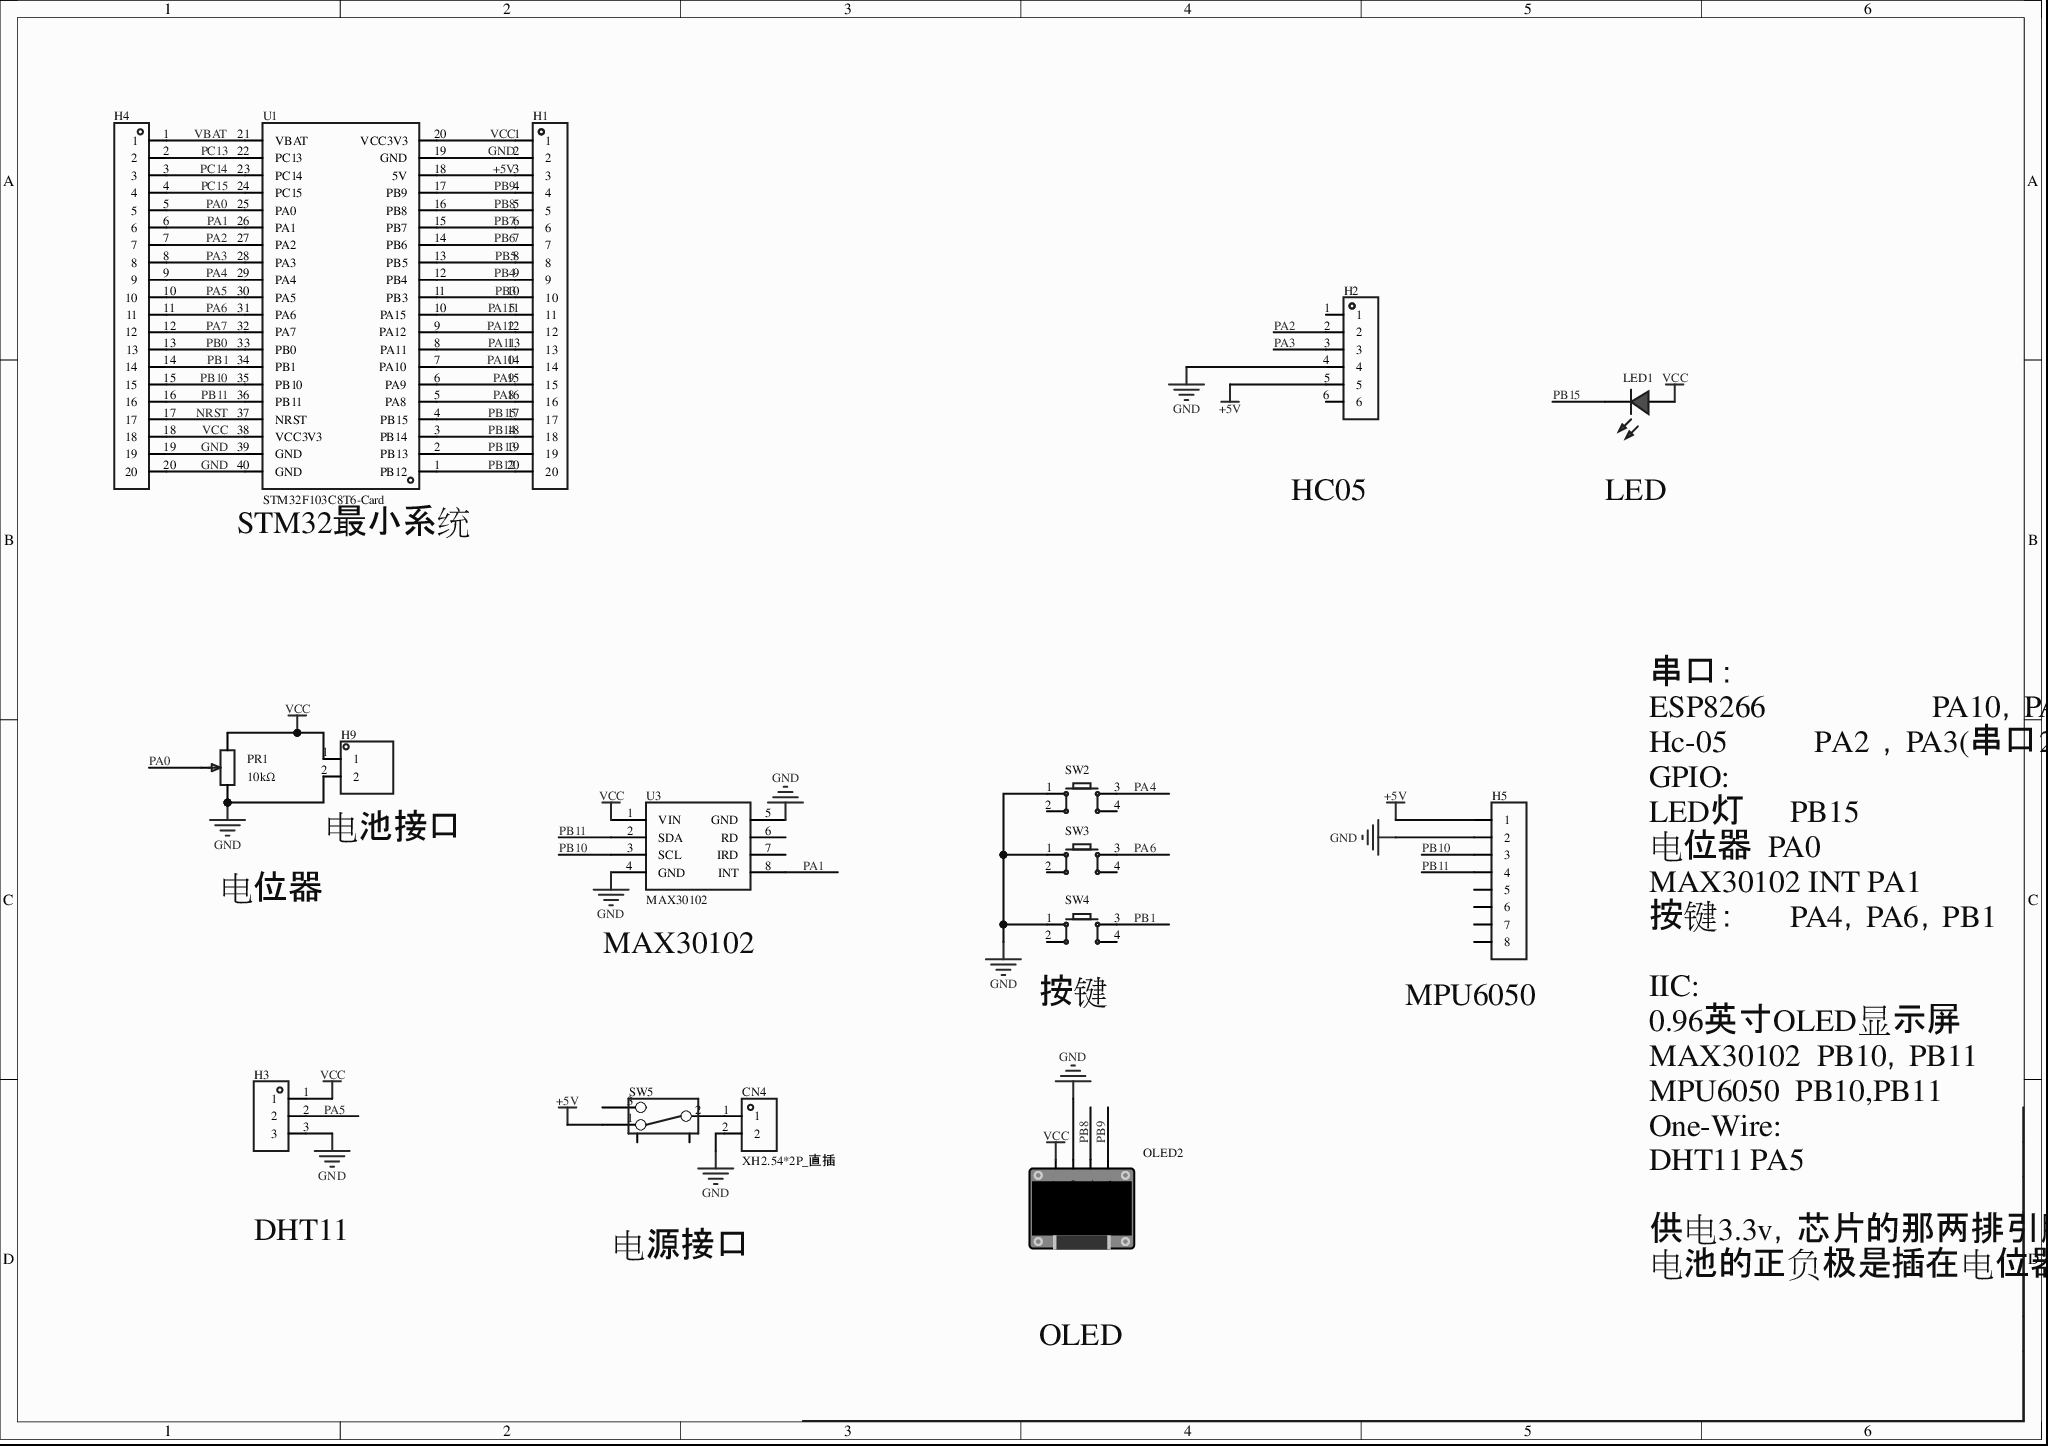
[diagram p0: MISC51261-3.schdoc]
# Altium project MISC51261-2.PrjPcb
1 sheet, 16 parts. Net scope: global (net labels, ports and power ports of the same name join across sheets).
Board file: MISC51261.pcbdoc

## Sheet MISC51261-3.schdoc
size 297 x 209 mm; Version: V1.0; @Project Name: MISC51261; @Page Count: 1; @Update Date: 2026-05-06; @Create Date: 2026-05-06; @Schematic Name: MISC51261; @Page No: 1; @Create Time: 23:22:16; @Update Time: 17:32:40; @Board Name: MISC51261

### Parts
CN4  XH2.54*2P_直插  [CONN-TH_2P-P2.50-XH2.54-2P]
H1  (no value)  [HDR-TH_20P-P2.54-V-M-1]
H2  (no value)  [HDR-TH_6P-P2.54-V-F]
H3  (no value)  [HDR-TH_3P-P2.54-V-F]
H4  (no value)  [HDR-TH_20P-P2.54-V-M-1]
H5  (no value)  [HDR-TH_8P-P2.54-V-F-1]
H9  (no value)  [HDR-TH_2P-P2.54-V-M-1]
LED1  (no value)  [LED_TH-3mm]
OLED2  (no value)  [0.96OLED_4P]
PR1  10kΩ  [R_3296]
SW2  (no value)  [SW-TH_4P-L6.0-W6.0-P4.50-LS6.5]
SW3  (no value)  [SW-TH_4P-L6.0-W6.0-P4.50-LS6.5]
SW4  (no value)  [SW-TH_4P-L6.0-W6.0-P4.50-LS6.5]
SW5  (no value)  [拨动开关]
U1  STM32F103C8T6-Card  [CONN-TH_L53.3-W22.9_STM32F103C8T6-CARD]
U3  MAX30102  [MAX30102]

### Nets
+5V: H1.3 H2.5 H5.1 SW5.1 U1.18(5V)
GND: CN4.2 H1.2 H2.4 H3.3 H4.19 H4.20 H5.2 H9.2 OLED2.2(GND) PR1.3 SW2.1 SW3.1 SW4.1 U1.19(GND) U1.39(GND) U1.40(GND) U3.4(GND) U3.5(GND)
VCC: H1.1 H3.1 H4.18 H9.1 LED1.1(C) OLED2.1(VCC) PR1.1 U1.20(VCC3V3) U1.38(VCC3V3) U3.1(VIN)
NRST: H4.17 U1.37(NRST)
PA0: H4.5 PR1.2 U1.25(PA0)
PA1: H4.6 U1.26(PA1) U3.8(INT)
PA2: H2.2 H4.7 U1.27(PA2)
PA3: H2.3 H4.8 U1.28(PA3)
PA4: H4.9 SW2.3 U1.29(PA4)
PA5: H3.2 H4.10 U1.30(PA5)
PA6: H4.11 SW3.3 U1.31(PA6)
PA7: H4.12 U1.32(PA7)
PA8: H1.16 U1.5(PA8)
PA9: H1.15 U1.6(PA9)
PA10: H1.14 U1.7(PA10)
PA11: H1.13 U1.8(PA11)
PA12: H1.12 U1.9(PA12)
PA15: H1.11 U1.10(PA15)
PB0: H4.13 U1.33(PB0)
PB1: H4.14 SW4.3 U1.34(PB1)
PB3: H1.10 U1.11(PB3)
PB4: H1.9 U1.12(PB4)
PB5: H1.8 U1.13(PB5)
PB6: H1.7 U1.14(PB6)
PB7: H1.6 U1.15(PB7)
PB8: H1.5 OLED2.3(SCL) U1.16(PB8)
PB9: H1.4 OLED2.4(SDA) U1.17(PB9)
PB10: H4.15 H5.3 U1.35(PB10) U3.3(SCL)
PB11: H4.16 H5.4 U1.36(PB11) U3.2(SDA)
PB12: H1.20 U1.1(PB12)
PB13: H1.19 U1.2(PB13)
PB14: H1.18 U1.3(PB14)
PB15: H1.17 LED1.2(A) U1.4(PB15)
PC13: H4.2 U1.22(PC13)
PC14: H4.3 U1.23(PC14)
PC15: H4.4 U1.24(PC15)
VBAT: H4.1 U1.21(VBAT)
NetCN4_1: CN4.1 SW5.2

Not connected (* = marked no-connect by the designer): H2 1 6; H5 5 6 7 8; SW2 2 4; SW3 2 4; SW4 2 4; SW5 3 4 5; U3 6(RD) 7(IRD)

### Notes on the sheet
- HC05
- LED
- (near U1) STM32最小系统
- 串口：
  ESP8266  		PA10，PA9 	(串口1）
  Hc-05           PA2  ，PA3(串口2)
  GPIO:
  LED灯	PB15
  电位器  PA0
  MAX30102 INT PA1
  按键：	PA4，PA6，PB1
  IIC:
  0.96英寸OLED显示屏	PB8，PB9
  MAX30102  PB10，PB11
  MPU6050  PB10,PB11
  One-Wire:
  DHT11 PA5
  供电3.3v，芯片的那两排引脚整两排我能插杜邦线的
  电池的正负极是插在电位器的两端的
- (near H9) 电池接口
- 电位器
- (near U3) MAX30102
- (near SW4) 按键
- (near H5) MPU6050
- DHT11
- 电源接口
- OLED

### Library data of the parts
CN4 = XH2.54*2P_直插: 3D Model: 325c595e30db4df8abe76612dd40b0fa0819f05c4eef4c71ace90d822a990e87; 3D Model Transform: 295.275,228.346,0,180,0,0,-0.002,-20.079,-137.795; AddInBom: yes; Device: XH2.54*2P_直插; Symbol: XH2.54*2P_直插; LCSC Part Name: XH2.54*2P_直插; Supplier Part: C9900008615; Manufacturer Part: XH2.54*2P_直插; Supplier Footprint: XH2.54_2P; JLCPCB Part Class: Extended Part; Supplier: LCSC; FootprintName: CONN-TH_2P-P2.50-XH2.54-2P; ConvertToPcb: yes; ModelName: CONN-TH_2P-P2.50-XH2.54-2P
H1 H4 = HDR-M_2.54_1x20P: 间距:2.54mm;总PIN位数:20;排数:1;插针结构:-;行距:-;安装类型:直插;圆针/方针:-;额定电流:-;额定电压:-;配合针长度:-;塑高:-;触头材质:黄铜;触头镀层:-;颜色:黑色;; Symbol: HDR_2.54-1x20P; ConvertToPcb: yes; ModelId: f68709be121d406db68b06f32a5953890819f05c4eef4c71ace90d822a990e87; ModelName: HDR-M-2.54_1x20; ModelTransform: 1999.996,100,0,0,0,0,0,0,-118.11; Device: HDR-M_2.54_1x20P; AddInBom: yes; SupplierPart: C50981; Supplier Footprint: 插件; FootprintName: HDR-TH_20P-P2.54-V-M-1
H2 = HDR-F_2.54_1x6P: Symbol: Header-Female-2.54_1x6; ConvertToPcb: yes; ModelId: 0f5bcf94dcda47d085f24cdca1696fe9; ModelTransform: 619.684,94.488,0,0,0,0,0,0,-125.984; Device: HDR-F_2.54_1x6P; AddInBom: yes; SupplierPart: C40877; Supplier Footprint: 插件; FootprintName: HDR-TH_6P-P2.54-V-F; ModelName: HDR-TH_6P-P2.54-V-F
H3 = HDR-F_2.54_1x3P: Symbol: PM254V-11-03-H85; 3D Model: f3b3cc5aae9641bf9e56fc160cef875b; 3D Model Transform: 299.9994,100,0,0,0,0,0,0,-118.11; ConvertToPcb: yes; ModelName: HDR2.54-F-LI-1X3P; Device: HDR-F_2.54_1x3P; Supplier Part: C541850; Supplier Footprint: 插件; FootprintName: HDR-TH_3P-P2.54-V-F; AddInBom: yes
H5 = HDR-F_2.54_1x8P: Symbol: Header-Female-2.54_1x8; AddInBom: yes; ModelId: 0f7e4d9227ef4fa08d5469c22cc70cdb; ModelName: HDR-F-2.54_1x8; ModelTransform: 799.99844,100,0,0,0,0,0,0,-118.11; Device: HDR-F_2.54_1x8P; ConvertToPcb: yes; FootprintName: HDR-TH_8P-P2.54-V-F-1; SupplierPart: C27438; Supplier Footprint: 插件
H9 = HDR-M_2.54_1x2P: Symbol: 210S-1*2P L=11.6MMGold-plated black; ConvertToPcb: yes; ModelId: 79b2e9f2d70a4d68a1b7098f27c6d4c50819f05c4eef4c71ace90d822a990e87; ModelName: HDR-M-2.54_1x2; ModelTransform: 200,100,0,0,0,0,0,0,-118.11; Device: HDR-M_2.54_1x2P; AddInBom: yes; SupplierPart: C124375; Supplier Footprint: 插件; FootprintName: HDR-TH_2P-P2.54-V-M-1
LED1 = LED_TH-R_3mm: 3D Model: a497c992633541038a38947cdc58012f0819f05c4eef4c71ace90d822a990e87; 3D Model Transform: 141.274,153.327,0,0,0,0,-5.984,0,-137.795; ConvertToPcb: yes; ModelName: LED-TH-3mm_R; Symbol: LED_TH-R; Device: LED_TH-R_3mm; Supplier Footprint: 插件; AddInBom: yes; FootprintName: LED_TH-3mm
OLED2 = 0.96OLED模块_4P: Symbol: 0.96OLED模块_4P_1; 3D Model: 79c000fdb68d45a296c2e9bedf4f9055; 3D Model Transform: 1393.69792,1318.895,0,0,0,0,0,-560.079,-137.795; ConvertToPcb: yes; Device: 0.96OLED模块_4P; Supplier Footprint: 插件; AddInBom: yes; FootprintName: 0.96OLED_4P; ModelName: 0.96OLED_4P
PR1 = R_3296: ConvertToPcb: yes; ModelId: b182808559bb43bda9e7de64b64134cb; ModelName: 3296W; ModelTransform: 373.98,188.96,590.49,180,0,0,0,0,-140; Symbol: R_3296; Device: R_3296; AddInBom: yes; Supplier Footprint: 直插; FootprintName: R_3296; Value: 10kΩ
SW2-SW4 = Key_TH_6x6x6: 触点电流:50mA;额定电压(DC):12V;绝缘电阻:100MΩ;电路结构:单刀单掷;安装方式:直插;按钮形状:圆形按钮;按钮/盖帽颜色:黑色;作用力:260gf@±30gf;工作温度:-25℃~+70℃;引脚样式:PC引脚;开关长度:6mm;开关宽度:6mm;开关高度:6mm;带支架:否;; Symbol: 轻触按键; AddInBom: yes; ModelId: 20eee248bc684ccd8cbdbb1d0d91ec6f0819f05c4eef4c71ace90d822a990e87; ModelName: SW-TH_4P-L6.0-W6.0-H5.0-LS6.5-P4.50; ModelTransform: 236.22,323.03,0,90,0,0,0,0,-137.795; Device: Key_TH_6x6x6; FootprintName: SW-TH_4P-L6.0-W6.0-P4.50-LS6.5; ConvertToPcb: yes; Supplier Footprint: 插件
SW5 = 拨动开关_正: ConvertToPcb: yes; ModelId: 4321fe59a4074cbfb4989553f297c68f0819f05c4eef4c71ace90d822a990e87; ModelName: SW-TH_SS-12D02-VG4; ModelTransform: 370.09,208.7,472.35,0,0,0,0,0,-110; Device: 拨动开关_正; Symbol: 拨动开关; FootprintName: 拨动开关; AddInBom: yes; Supplier Footprint: 插件
U1 = STM32F103C8T6-Card: AddInBom: yes; Device: STM32F103C8T6-Card; Symbol: STM32F103C8T6-CARD; FootprintName: CONN-TH_L53.3-W22.9_STM32F103C8T6-CARD; LCSC Part Name: STM32F103C8T6-Card; SupplierPart: C9900077949; ManufacturerPart: STM32F103C8T6-Card; Supplier Footprint: 插件; Supplier: LCSC; ConvertToPcb: yes
U3 = MAX30102: AddInBom: yes; Symbol: MAX30102; Device: MAX30102; ConvertToPcb: yes; FootprintName: MAX30102